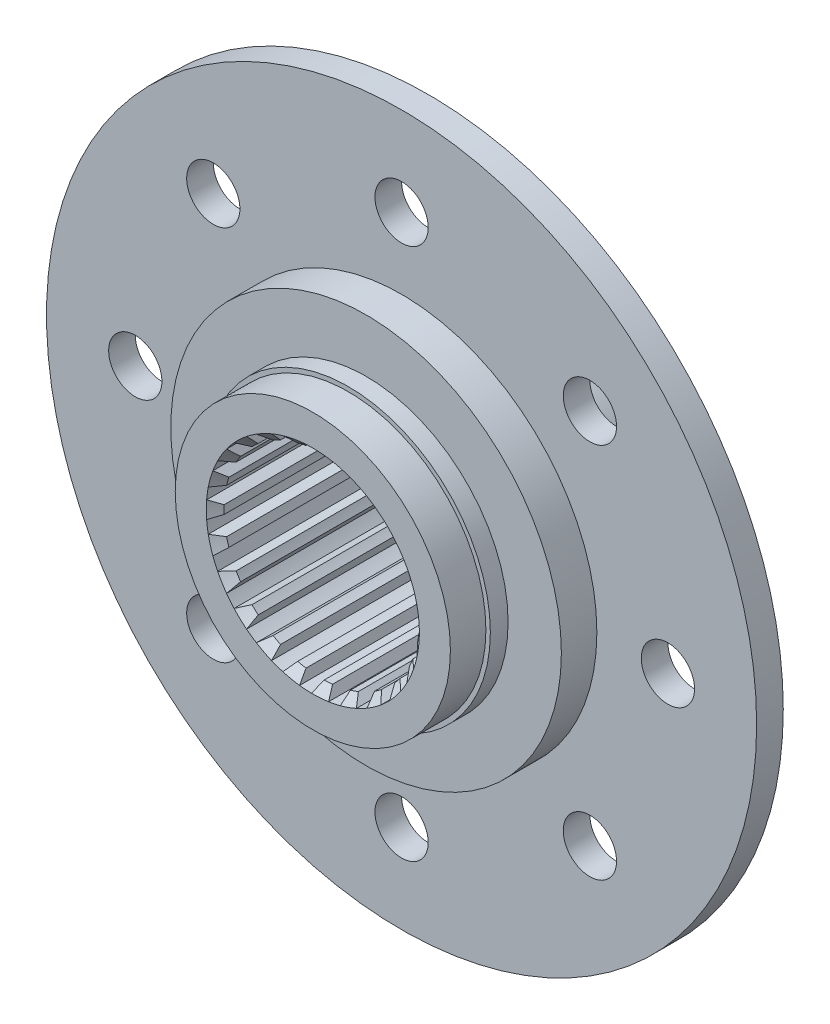
SolidWorks part; units mm, degrees
ref_plane "Front Plane" through (0, 0, 0) normal (0, 0, 1) x (1, 0, 0)
ref_plane "Top Plane" through (0, 0, 0) normal (0, 1, 0) x (1, 0, 0)
ref_plane "Right Plane" through (0, 0, 0) normal (1, 0, 0) x (0, 0, -1)
other "Configuration Table"
sketch "Sketch1" plane through (0, 0, 0) normal (0, 0, 1) x (1, 0, 0)
  circle A0 centre (0, 0) radius 40
extrude "Boss-Extrude1" add sketch "Sketch1" along normal blind 3
sketch "Sketch2" plane through (0, 0, 0) normal (0, 0, -1) x (-1, 0, 0)
  circle A0 centre (0, 0) radius 18
extrude "Boss-Extrude2" add sketch "Sketch2" along normal blind 1
sketch "Sketch3" plane through (0, 0, -1) normal (0, 0, -1) x (-1, 0, 0)
  circle A0 centre (0, 0) radius 16
extrude "Boss-Extrude3" add sketch "Sketch3" along normal blind 3
sketch "Sketch4" plane through (0, 0, -4) normal (0, 0, -1) x (-1, 0, 0)
  circle A0 centre (0, 0) radius 15.5
extrude "Boss-Extrude4" add sketch "Sketch4" along normal blind 9
sketch "Sketch5" plane through (0, 0, 3) normal (0, 0, 1) x (1, 0, 0)
  circle A0 centre (0, 0) radius 22
extrude "Boss-Extrude5" add sketch "Sketch5" along normal blind 4
sketch "Sketch6" plane through (0, 0, 7) normal (0, 0, 1) x (1, 0, 0)
  circle A0 centre (0, 0) radius 16
extrude "Boss-Extrude6" add sketch "Sketch6" along normal blind 2
sketch "Sketch7" plane through (0, 0, 9) normal (0, 0, 1) x (1, 0, 0)
  circle A0 centre (0, 0) radius 15.5
extrude "Boss-Extrude7" add sketch "Sketch7" along normal blind 4
sketch "Sketch8" plane through (0, 0, 0) normal (0, 0, -1) x (-1, 0, 0)
  circle A0 centre (0, 0) radius 30 construction
  circle A1 centre (0, 30) radius 3
  circle A2 centre (21.2132, 21.2132) radius 3
  circle A3 centre (30, 0) radius 3
  circle A4 centre (21.2132, -21.2132) radius 3
  circle A5 centre (0, -30) radius 3
  circle A6 centre (-21.2132, -21.2132) radius 3
  circle A7 centre (-30, 0) radius 3
  circle A8 centre (-21.2132, 21.2132) radius 3
  point P22 (0, 0)
  dimension "D1" = 8
extrude "Cut-Extrude1" cut sketch "Sketch8" against normal blind 12
sketch "Sketch10" plane through (0, 0, -13) normal (0, 0, -1) x (-1, 0, 0)
  circle A0 centre (0, 0) radius 12
extrude "Cut-Extrude2" cut sketch "Sketch10" against normal blind 33
sketch "Sketch11" plane through (0, 0, -13) normal (0, 0, -1) x (-1, 0, 0)
  line L0 (-11.7187, 2.5831) -> (-10.8223, 1.9695)
  line L1 (-11.981, 0.6744) -> (-10.9523, 1.0234)
  line L2 (-10.5872, 5.6489) -> (-9.8896, 4.8162)
  line L3 (-11.3548, 3.8818) -> (-10.27, 3.9403)
  line L4 (-8.6706, 8.2959) -> (-8.2234, 7.3058)
  line L5 (-9.8864, 6.8014) -> (-8.8261, 6.565)
  line L6 (-6.1108, 10.3275) -> (-5.9474, 9.2536)
  line L7 (-7.6848, 9.2165) -> (-6.7276, 8.7028)
  line L8 (-3.0979, 11.5932) -> (-3.2303, 10.515)
  line L9 (-4.9133, 10.948) -> (-4.1301, 10.1952)
  line L10 (0.1448, 11.9991) -> (-0.2736, 10.9966)
  line L11 (-1.7773, 11.8676) -> (-1.2263, 10.9314)
  line L12 (3.3768, 11.5151) -> (2.7034, 10.6626)
  line L13 (1.4904, 11.9071) -> (1.7684, 10.8569)
  line L14 (6.3583, 10.177) -> (5.4799, 9.5379)
  line L15 (4.6476, 11.0634) -> (4.632, 9.9772)
  line L16 (8.8682, 8.0842) -> (7.85, 7.7057)
  line L17 (7.4602, 9.3992) -> (7.152, 8.3575)
  line L18 (10.7205, 5.3918) -> (9.6379, 5.3021)
  line L19 (9.7194, 7.038) -> (9.1417, 6.118)
  line L20 (11.7776, 2.2995) -> (10.7109, 2.5052)
  line L21 (11.2578, 4.1547) -> (10.4533, 3.4248)
  line L22 (11.9613, -0.9633) -> (10.9896, -0.4775)
  line L23 (11.9613, 0.9633) -> (10.9896, 0.4775)
  line L24 (11.2578, -4.1547) -> (10.4533, -3.4248)
  line L25 (11.7776, -2.2995) -> (10.7109, -2.5052)
  line L26 (9.7194, -7.038) -> (9.1417, -6.118)
  line L27 (10.7205, -5.3918) -> (9.6379, -5.3021)
  line L28 (7.4602, -9.3992) -> (7.152, -8.3575)
  line L29 (8.8682, -8.0842) -> (7.85, -7.7057)
  line L30 (4.6476, -11.0634) -> (4.632, -9.9772)
  line L31 (6.3583, -10.177) -> (5.4799, -9.5379)
  line L32 (1.4904, -11.9071) -> (1.7684, -10.8569)
  line L33 (3.3768, -11.5151) -> (2.7034, -10.6626)
  line L34 (-1.7773, -11.8676) -> (-1.2263, -10.9314)
  line L35 (0.1448, -11.9991) -> (-0.2736, -10.9966)
  line L36 (-4.9133, -10.948) -> (-4.1301, -10.1952)
  line L37 (-3.0979, -11.5932) -> (-3.2303, -10.515)
  line L38 (-7.6848, -9.2165) -> (-6.7276, -8.7028)
  line L39 (-6.1108, -10.3275) -> (-5.9474, -9.2536)
  line L40 (-9.8864, -6.8014) -> (-8.8261, -6.565)
  line L41 (-8.6706, -8.2959) -> (-8.2234, -7.3058)
  line L42 (-11.3548, -3.8818) -> (-10.27, -3.9403)
  line L43 (-10.5872, -5.6489) -> (-9.8896, -4.8162)
  line L44 (-11.981, -0.6744) -> (-10.9523, -1.0234)
  line L45 (-11.7187, -2.5831) -> (-10.8223, -1.9695)
  arc A0 (-10.8223, 1.9695) -> (-10.9523, 1.0234) centre (0, 0) ccw
  circle A1 centre (0, 0) radius 12 construction
  arc A2 (-11.7187, 2.5831) -> (-11.981, 0.6744) centre (0, 0) ccw
  arc A3 (-9.8896, 4.8162) -> (-10.27, 3.9403) centre (0, 0) ccw
  arc A4 (-10.5872, 5.6489) -> (-11.3548, 3.8818) centre (0, 0) ccw
  arc A5 (-8.2234, 7.3058) -> (-8.8261, 6.565) centre (0, 0) ccw
  arc A6 (-8.6706, 8.2959) -> (-9.8864, 6.8014) centre (0, 0) ccw
  arc A7 (-5.9474, 9.2536) -> (-6.7276, 8.7028) centre (0, 0) ccw
  arc A8 (-6.1108, 10.3275) -> (-7.6848, 9.2165) centre (0, 0) ccw
  arc A9 (-3.2303, 10.515) -> (-4.1301, 10.1952) centre (0, 0) ccw
  arc A10 (-3.0979, 11.5932) -> (-4.9133, 10.948) centre (0, 0) ccw
  arc A11 (-0.2736, 10.9966) -> (-1.2263, 10.9314) centre (0, 0) ccw
  arc A12 (0.1448, 11.9991) -> (-1.7773, 11.8676) centre (0, 0) ccw
  arc A13 (2.7034, 10.6626) -> (1.7684, 10.8569) centre (0, 0) ccw
  arc A14 (3.3768, 11.5151) -> (1.4904, 11.9071) centre (0, 0) ccw
  arc A15 (5.4799, 9.5379) -> (4.632, 9.9772) centre (0, 0) ccw
  arc A16 (6.3583, 10.177) -> (4.6476, 11.0634) centre (0, 0) ccw
  arc A17 (7.85, 7.7057) -> (7.152, 8.3575) centre (0, 0) ccw
  arc A18 (8.8682, 8.0842) -> (7.4602, 9.3992) centre (0, 0) ccw
  arc A19 (9.6379, 5.3021) -> (9.1417, 6.118) centre (0, 0) ccw
  arc A20 (10.7205, 5.3918) -> (9.7194, 7.038) centre (0, 0) ccw
  arc A21 (10.7109, 2.5052) -> (10.4533, 3.4248) centre (0, 0) ccw
  arc A22 (11.7776, 2.2995) -> (11.2578, 4.1547) centre (0, 0) ccw
  arc A23 (10.9896, -0.4775) -> (10.9896, 0.4775) centre (0, 0) ccw
  arc A24 (11.9613, -0.9633) -> (11.9613, 0.9633) centre (0, 0) ccw
  arc A25 (10.4533, -3.4248) -> (10.7109, -2.5052) centre (0, 0) ccw
  arc A26 (11.2578, -4.1547) -> (11.7776, -2.2995) centre (0, 0) ccw
  arc A27 (9.1417, -6.118) -> (9.6379, -5.3021) centre (0, 0) ccw
  arc A28 (9.7194, -7.038) -> (10.7205, -5.3918) centre (0, 0) ccw
  arc A29 (7.152, -8.3575) -> (7.85, -7.7057) centre (0, 0) ccw
  arc A30 (7.4602, -9.3992) -> (8.8682, -8.0842) centre (0, 0) ccw
  arc A31 (4.632, -9.9772) -> (5.4799, -9.5379) centre (0, 0) ccw
  arc A32 (4.6476, -11.0634) -> (6.3583, -10.177) centre (0, 0) ccw
  arc A33 (1.7684, -10.8569) -> (2.7034, -10.6626) centre (0, 0) ccw
  arc A34 (1.4904, -11.9071) -> (3.3768, -11.5151) centre (0, 0) ccw
  arc A35 (-1.2263, -10.9314) -> (-0.2736, -10.9966) centre (0, 0) ccw
  arc A36 (-1.7773, -11.8676) -> (0.1448, -11.9991) centre (0, 0) ccw
  arc A37 (-4.1301, -10.1952) -> (-3.2303, -10.515) centre (0, 0) ccw
  arc A38 (-4.9133, -10.948) -> (-3.0979, -11.5932) centre (0, 0) ccw
  arc A39 (-6.7276, -8.7028) -> (-5.9474, -9.2536) centre (0, 0) ccw
  arc A40 (-7.6848, -9.2165) -> (-6.1108, -10.3275) centre (0, 0) ccw
  arc A41 (-8.8261, -6.565) -> (-8.2234, -7.3058) centre (0, 0) ccw
  arc A42 (-9.8864, -6.8014) -> (-8.6706, -8.2959) centre (0, 0) ccw
  arc A43 (-10.27, -3.9403) -> (-9.8896, -4.8162) centre (0, 0) ccw
  arc A44 (-11.3548, -3.8818) -> (-10.5872, -5.6489) centre (0, 0) ccw
  arc A45 (-10.9523, -1.0234) -> (-10.8223, -1.9695) centre (0, 0) ccw
  arc A46 (-11.981, -0.6744) -> (-11.7187, -2.5831) centre (0, 0) ccw
  point P97 (0, 0)
  dimension "D1" = 23
extrude "Boss-Extrude8" add sketch "Sketch11" against normal up to surface (26 mm away) up to face at (12, 0, 13)
sketch "Sketch12" plane through (0, 0, 0) normal (0, 1, 0) x (1, 0, 0)
  line L0 (0, 13) -> (-12, 13)
  line L1 (15.5, 13) -> (-15.5, 13) construction
  line L2 (-8.5105, 11) -> (0, 11)
  line L3 (-12, 13) -> (-10, 11)
  line L5 (-10, 11) -> (-8.5105, 11)
  line L6 (0, 11) -> (0, 13)
  line L7 (0, 0) -> (-23.3962, 0) construction
  line L8 (40, 0) -> (-40, 0) construction
  line L9 (0, -11) -> (0, -13)
  line L10 (-10, -11) -> (-8.5105, -11)
  line L11 (-12, -13) -> (-10, -11)
  line L12 (-8.5105, -11) -> (0, -11)
  line L13 (0, -13) -> (-12, -13)
revolve "Cut-Revolve1" cut sketch "Sketch12" angle 360 about L6
